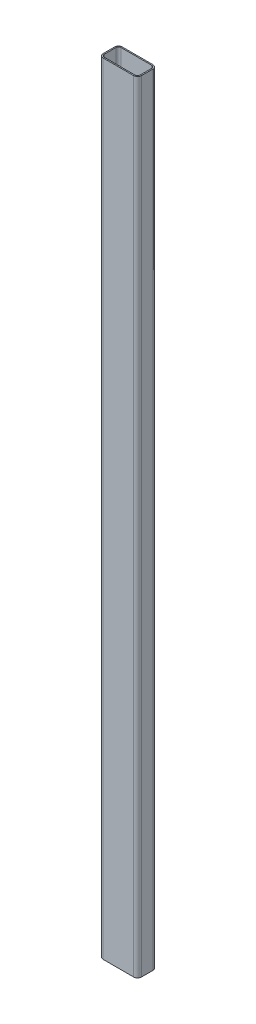
from build123d import *

# Parameters (mm, degrees)
EXTRUDE_THIN1_DEPTH = 1020


with BuildPart() as part:
    # Sketch1 → Extrude-Thin1 (new, symmetric)
    with BuildSketch(Plane(origin=(0, 0, 0), x_dir=(1, 0, 0), z_dir=(0, 1, 0))):
        with BuildLine():
            Line((-40, 25), (40, 25))
            ThreePointArc((40, 25), (47.071067812, 22.071067812), (50, 15))
            Line((50, 15), (50, -15))
            ThreePointArc((50, -15), (47.071067812, -22.071067812), (40, -25))
            Line((40, -25), (-40, -25))
            ThreePointArc((-40, -25), (-47.071067812, -22.071067812), (-50, -15))
            Line((-50, -15), (-50, 15))
            ThreePointArc((-50, 15), (-47.071067812, 22.071067812), (-40, 25))
        make_face()
        with BuildLine():
            Line((-40, 22), (40, 22))
            ThreePointArc((40, 22), (44.949747468, 19.949747468), (47, 15))
            Line((47, 15), (47, -15))
            ThreePointArc((47, -15), (44.949747468, -19.949747468), (40, -22))
            Line((40, -22), (-40, -22))
            ThreePointArc((-40, -22), (-44.949747468, -19.949747468), (-47, -15))
            Line((-47, -15), (-47, 15))
            ThreePointArc((-47, 15), (-44.949747468, 19.949747468), (-40, 22))
        make_face(mode=Mode.SUBTRACT)
    extrude(amount=EXTRUDE_THIN1_DEPTH, both=True)


solid = part.part
